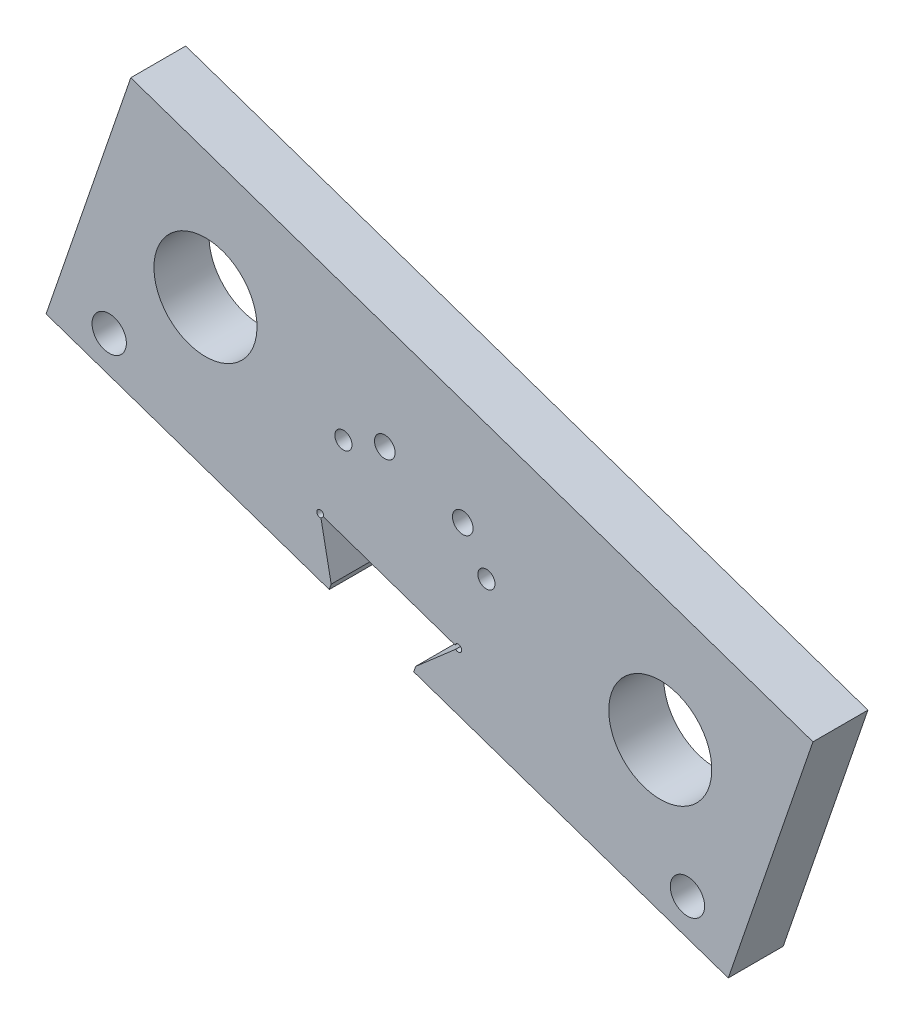
SolidWorks part; units mm, degrees
ref_plane "前视基准面" through (0, 0, 0) normal (0, 0, 1) x (1, 0, 0)
ref_plane "上视基准面" through (0, 0, 0) normal (0, 1, 0) x (1, 0, 0)
ref_plane "右视基准面" through (0, 0, 0) normal (1, 0, 0) x (0, 0, -1)
sketch "草图1" plane through (0, 0, 0) normal (0, 0, 1) x (1, 0, 0)
  line L0 (-128.9517, 174.8902) -> (-228.2697, 208.9627) construction
  line L2 (-123.2729, 191.4432) -> (-134.6304, 158.3372)
  line L3 (-222.5909, 225.5157) -> (-233.9484, 192.4097)
  line L4 (-123.2729, 191.4432) -> (-222.5909, 225.5157)
  line L6 (-134.6304, 158.3372) -> (-233.9484, 192.4097)
  circle A0 centre (-211.7167, 203.2839) radius 7.5 construction
  circle A1 centre (-145.5047, 180.5689) radius 7.5 construction
  circle A2 centre (-211.7167, 203.2839) radius 7.5
  circle A3 centre (-145.5047, 180.5689) radius 7.5
  point P6 (-145.5047, 180.5689)
  point P7 (-194.2167, 203.2839)
  point P8 (-211.7167, 203.2839)
  point P14 (-128.0047, 180.5689)
extrude "凸台-拉伸1" add sketch "草图1" along normal up to surface (8 mm away)
sketch "草图2" plane through (34.4234, 100.3408, 0) normal (-0.3245, -0.9459, 0) x (0.9459, -0.3245, 0)
  line L4 (-178.7254, 0) -> (-178.7254, 8)
  line L5 (-178.7254, 8) -> (-283.7254, 8)
  line L6 (-283.7254, 8) -> (-283.7254, 0)
  line L7 (-283.7254, 0) -> (-178.7254, 0)
  line L8 (-178.7254, 0) -> (-178.7254, 8)
  line L9 (-178.7254, 8) -> (-283.7254, 8)
  line L10 (-283.7254, 8) -> (-283.7254, 0)
  line L11 (-283.7254, 0) -> (-178.7254, 0)
  dimension "D1" = 0
extrude "凸台-拉伸2" add sketch "草图2" along normal blind 3
sketch "草图3" plane through (0, 0, 8) normal (0, 0, 1) x (1, 0, 0)
  line L2 (-135.6039, 155.4995) -> (-234.9219, 189.572) construction
  line L3 (-181.8738, 171.3731) -> (-193.2244, 175.2671)
  line L6 (-174.9089, 177.4414) -> (-194.9973, 184.333)
  line L7 (-181.8738, 171.3731) -> (-174.9089, 177.4414)
  line L8 (-193.2244, 175.2671) -> (-194.9973, 184.333)
  line L10 (-133.0079, 163.0666) -> (-232.3259, 197.1391) construction
  line L14 (-135.6039, 155.4995) -> (-234.9219, 189.572) construction
  point P0 (-182.5253, 187.964)
  point P1 (-187.5491, 173.3201)
  point P6 (-188.2006, 189.911)
  point P8 (-176.85, 186.017)
  dimension "D1" = 60
  dimension "D2" = 60
extrude "切除-拉伸1" cut sketch "草图3" against normal through all
hole_wizard "M6 螺纹孔1" positions "草图6" profile "草图5" tap size "M6" standard "GB"
sketch "草图6" plane through (0, 0, 8) normal (0, 0, 1) x (1, 0, 0)
  line L0 (-234.9219, 189.572) -> (-222.5909, 225.5157) construction
  line L1 (-193.2244, 175.2671) -> (-234.9219, 189.572) construction
  line L2 (-135.6039, 155.4995) -> (-181.8738, 171.3731) construction
  line L3 (-123.2729, 191.4432) -> (-135.6039, 155.4995) construction
  point P0 (-141.5485, 162.825)
  point P2 (-225.7323, 191.7055)
  dimension "D1" = 8
  dimension "D2" = 5
  dimension "D3" = 5
  dimension "D4" = 8
sketch "草图5" plane through (-141.5485, 162.825, 8) normal (1, 0, 0) x (0, -1, 0)
  line L0 (0, 0) -> (0, 16.5022)
  line L1 (0, 16.5022) -> (2.5, 15)
  line L2 (2.5, 15) -> (2.5, 0)
  line L5 (2.5, 0) -> (0, 0)
  line L10 (0, 16.5022) -> (-2.5, 15) construction
  line L11 (0, -6.35) -> (0, 107.95) construction
  dimension "螺纹孔钻头直径" = 5
  dimension "螺纹孔钻头深度" = 15
  dimension "导头角度" = 118
cosmetic thread "孔螺蚊线1" parameters "D1"=8, "D2"=6
cosmetic thread "孔螺蚊线2" parameters "D1"=8, "D2"=6
hole_wizard "M3 螺纹孔1" positions "草图7" profile "草图8" tap size "M3" standard "GB" end condition through all
sketch "草图7" plane through (0, 0, 0) normal (0, 0, -1) x (-1, 0, 0)
  point P0 (170.8192, 188.1883)
  point P2 (191.6356, 195.3069)
sketch "草图8" plane through (-170.8192, 188.1883, 0) normal (1, 0, 0) x (0, 1, 0)
  line L0 (0, 0) -> (0, 8)
  line L1 (0, 8) -> (1.25, 8)
  line L2 (1.25, 8) -> (1.25, 0)
  line L5 (1.25, 0) -> (0, 0)
  line L11 (0, -6.35) -> (0, 107.95) construction
  dimension "通孔螺纹孔钻头直径" = 2.5
  dimension "通孔螺纹孔钻头深度" = 8
cosmetic thread "孔螺蚊线3" parameters "D2"=3
cosmetic thread "孔螺蚊线4" parameters "D2"=3
hole_wizard "大小mm 暗销孔1" positions "草图11" profile "草图12" hole size "Ø3.0" standard "GB" end condition through all
sketch "草图11" plane through (0, 0, 0) normal (0, 0, -1) x (-1, 0, 0)
  point P0 (174.2562, 193.5902)
  point P2 (185.6106, 197.473)
sketch "草图12" plane through (-174.2562, 193.5902, 0) normal (1, 0, 0) x (0, 1, 0)
  line L0 (0, 0) -> (0, 8)
  line L1 (0, 8) -> (1.5, 8)
  line L2 (1.5, 8) -> (1.5, 0)
  line L5 (1.5, 0) -> (0, 0)
  line L11 (0, -6.35) -> (0, 107.95) construction
  dimension "通孔孔直径" = 3
  dimension "通孔孔深度" = 8
sketch "草图13" plane through (0, 0, 8) normal (0, 0, 1) x (1, 0, 0)
  line L2 (-193.6974, 175.4293) -> (-192.7321, 178.243)
  line L3 (-181.4008, 171.2108) -> (-180.8251, 172.8892)
  line L4 (-193.6974, 175.4293) -> (-181.4008, 171.2108)
  line L5 (-192.7321, 178.243) -> (-180.8251, 172.8892)
extrude "切除-拉伸2" cut sketch "草图13" against normal blind 10
sketch "草图14" plane through (0, 0, 8) normal (0, 0, 1) x (1, 0, 0)
  circle A0 centre (-194.9973, 184.333) radius 0.5
  circle A1 centre (-174.9089, 177.4414) radius 0.5
  dimension "D1" = 1
  dimension "D2" = 1
extrude "切除-拉伸3" cut sketch "草图14" against normal through all
